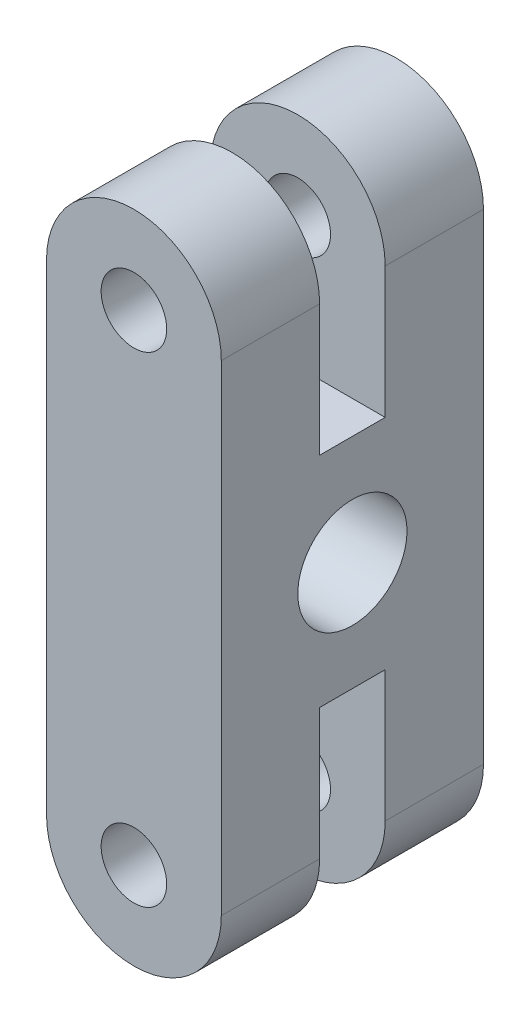
from build123d import *

# Parameters (mm, degrees)
BOSS_EXTRUDE1_DEPTH   = 12
SKETCH2_W             = 3
SKETCH2_H             = 20
CUT_EXTRUDE1_DEPTH    = 30.732137495
SKETCH3_R             = 1.5
CUT_EXTRUDE2_DEPTH    = 29.91366459
M6_TAPPED_HOLE1_D     = 5
M6_TAPPED_HOLE1_DEPTH = 6
M6_TAPPED_HOLE1_TIP   = 1.502151548


with BuildPart() as part:
    # Sketch1 → Boss-Extrude1 (new body)
    with BuildSketch(Plane.XY):
        with BuildLine():
            Line((-4, 0), (-4, 22))
            ThreePointArc((-4, 22), (0, 26), (4, 22))
            Line((4, 22), (4, 0))
            ThreePointArc((4, 0), (0, -4), (-4, 0))
        make_face()
    extrude(amount=BOSS_EXTRUDE1_DEPTH)

    # Sketch2 → Cut-Extrude1 (cut, through all)
    with BuildSketch(Plane.ZY.offset(4)):
        with Locations((6, 26)):
            Rectangle(SKETCH2_W, SKETCH2_H)
        with Locations((6, -4)):
            Rectangle(SKETCH2_W, SKETCH2_H)
    extrude(amount=-CUT_EXTRUDE1_DEPTH, mode=Mode.SUBTRACT)

    # Sketch3 → Cut-Extrude2 (cut, through all)
    with BuildSketch(Plane.XY.offset(12)):
        with Locations((0, 22)):
            Circle(SKETCH3_R)
        Circle(SKETCH3_R)
    extrude(amount=-CUT_EXTRUDE2_DEPTH, mode=Mode.SUBTRACT)

    # M6 Tapped Hole1
    with Locations(Plane(origin=(4, 11, 6), x_dir=(0, 0, 1), z_dir=(1, 0, 0))):
        with Locations((0, 0)):
            Hole(M6_TAPPED_HOLE1_D / 2, depth=M6_TAPPED_HOLE1_DEPTH)
            with Locations((0, 0, -(M6_TAPPED_HOLE1_DEPTH + M6_TAPPED_HOLE1_TIP / 2))):  # 118° drill point
                Cone(0, M6_TAPPED_HOLE1_D / 2, M6_TAPPED_HOLE1_TIP, mode=Mode.SUBTRACT)


solid = part.part
